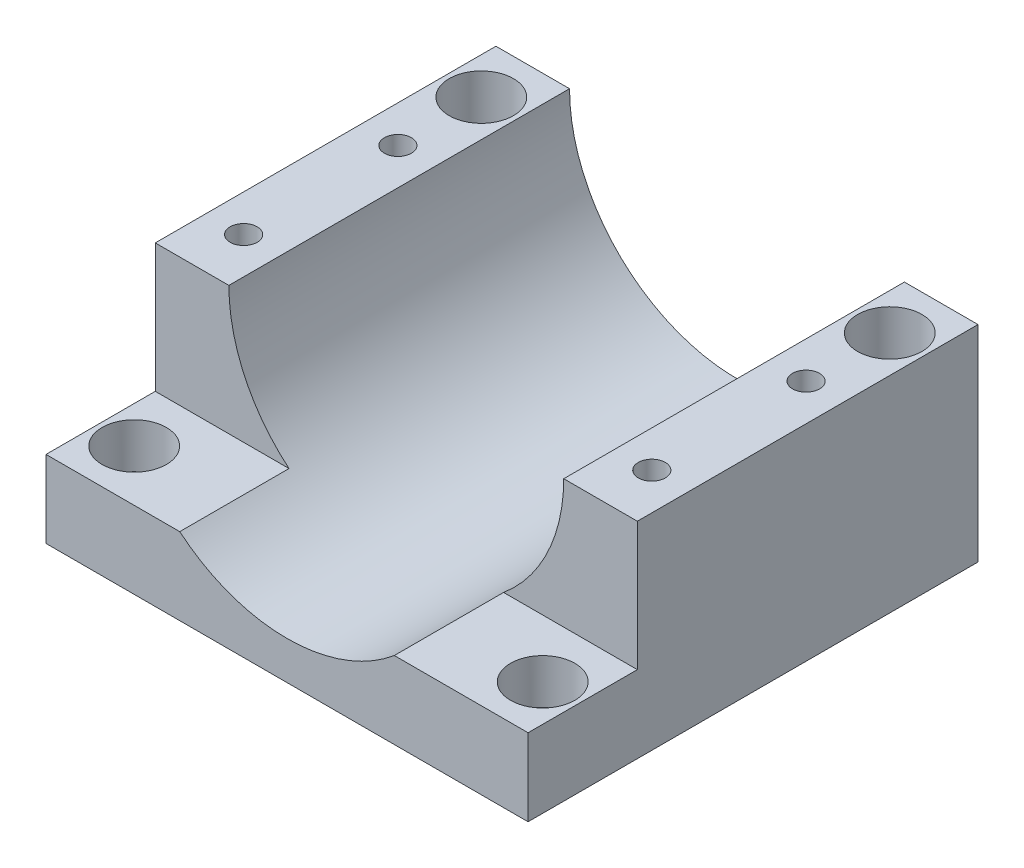
from build123d import *

# Parameters (mm, degrees)
SKETCH_2_W                   = 75
SKETCH_2_H                   = 32
EXTRUDE_1_DEPTH              = 70
SKETCH_4_R                   = 26.05
CUT_EXTRUDE_1_DEPTH          = 82.007715682
HOLE_WIZARD_M5_1_D           = 5.5
HOLE_WIZARD_M5_1_CBORE_D     = 10
HOLE_WIZARD_M5_1_CBORE_DEPTH = 27
SKETCH_7_W                   = 17
SKETCH_7_H                   = 20
CUT_EXTRUDE_2_DEPTH          = 104.831594421
HOLE_WIZARD_M5_1_2_D         = 4.2
HOLE_WIZARD_M5_1_2_DEPTH     = 12.4
HOLE_WIZARD_M5_1_2_TIP       = 1.2618073


with BuildPart() as part:
    # 草图2 → 凸台-拉伸1 (new body)
    with BuildSketch(Plane.XY):
        Rectangle(SKETCH_2_W, SKETCH_2_H)
    extrude(amount=EXTRUDE_1_DEPTH)

    # 草图4 → 切除-拉伸1 (cut, through all)
    with BuildSketch(Plane.XY.offset(70)):
        with Locations((0, 16)):
            Circle(SKETCH_4_R)
    extrude(amount=-CUT_EXTRUDE_1_DEPTH, mode=Mode.SUBTRACT)

    # Hole Wizard M5 _1 (through all)
    with Locations(Plane(origin=(0, 16, 0), x_dir=(1, 0, 0), z_dir=(0, 1, 0))):
        with Locations((-31.775, -8), (-31.775, -62), (31.775, -62), (31.775, -8)):
            CounterBoreHole(HOLE_WIZARD_M5_1_D / 2, HOLE_WIZARD_M5_1_CBORE_D / 2, HOLE_WIZARD_M5_1_CBORE_DEPTH)

    # 草图7 → 切除-拉伸2 (cut, through all)
    with BuildSketch(Plane.ZY.offset(37.5)):
        with Locations((61.5, 6)):
            Rectangle(SKETCH_7_W, SKETCH_7_H)
    extrude(amount=-CUT_EXTRUDE_2_DEPTH, mode=Mode.SUBTRACT)

    # Hole Wizard M5 _1 2
    with Locations(Plane(origin=(0, 16, 0), x_dir=(1, 0, 0), z_dir=(0, 1, 0))):
        with Locations((-31.75, -21), (-31.75, -45), (31.75, -21), (31.75, -45)):
            Hole(HOLE_WIZARD_M5_1_2_D / 2, depth=HOLE_WIZARD_M5_1_2_DEPTH)
            with Locations((0, 0, -(HOLE_WIZARD_M5_1_2_DEPTH + HOLE_WIZARD_M5_1_2_TIP / 2))):  # 118° drill point
                Cone(0, HOLE_WIZARD_M5_1_2_D / 2, HOLE_WIZARD_M5_1_2_TIP, mode=Mode.SUBTRACT)


solid = part.part
